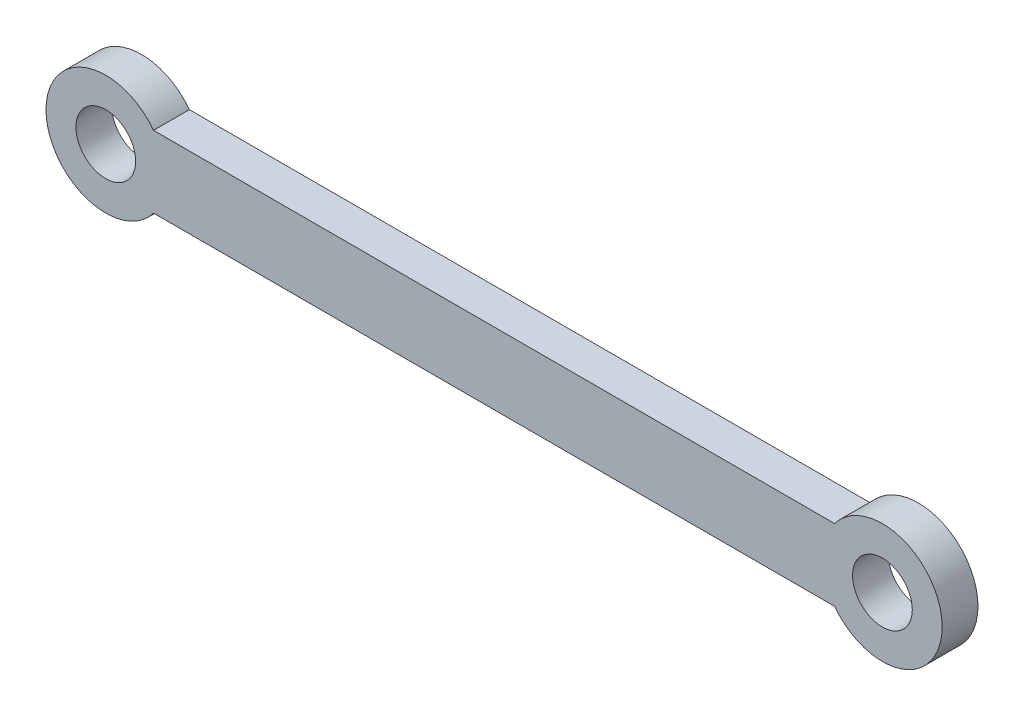
SolidWorks part; units mm, degrees
ref_plane "Front Plane" through (0, 0, 0) normal (0, 0, 1) x (1, 0, 0)
ref_plane "Top Plane" through (0, 0, 0) normal (0, 1, 0) x (1, 0, 0)
ref_plane "Right Plane" through (0, 0, 0) normal (1, 0, 0) x (0, 0, -1)
sketch "Sketch1" plane through (0, 0, 0) normal (0, 0, 1) x (1, 0, 0)
  line L2 (0, 0) -> (65, 0) construction
  line L3 (4, 3) -> (61, 3)
  line L4 (4, -3) -> (61, -3)
  circle A0 centre (0, 0) radius 2.5
  arc A1 (4, 3) -> (4, -3) centre (0, 0) ccw
  circle A2 centre (65, 0) radius 2.5
  arc A3 (61, -3) -> (61, 3) centre (65, 0) ccw
  dimension "D1" = 65
  dimension "D2" = 5
  dimension "D3" = 5
  dimension "D4" = 10
  dimension "D5" = 10
  dimension "D8" = 6
  dimension "D9" = 3
extrude "Boss-Extrude1" add sketch "Sketch1" along normal blind 3
